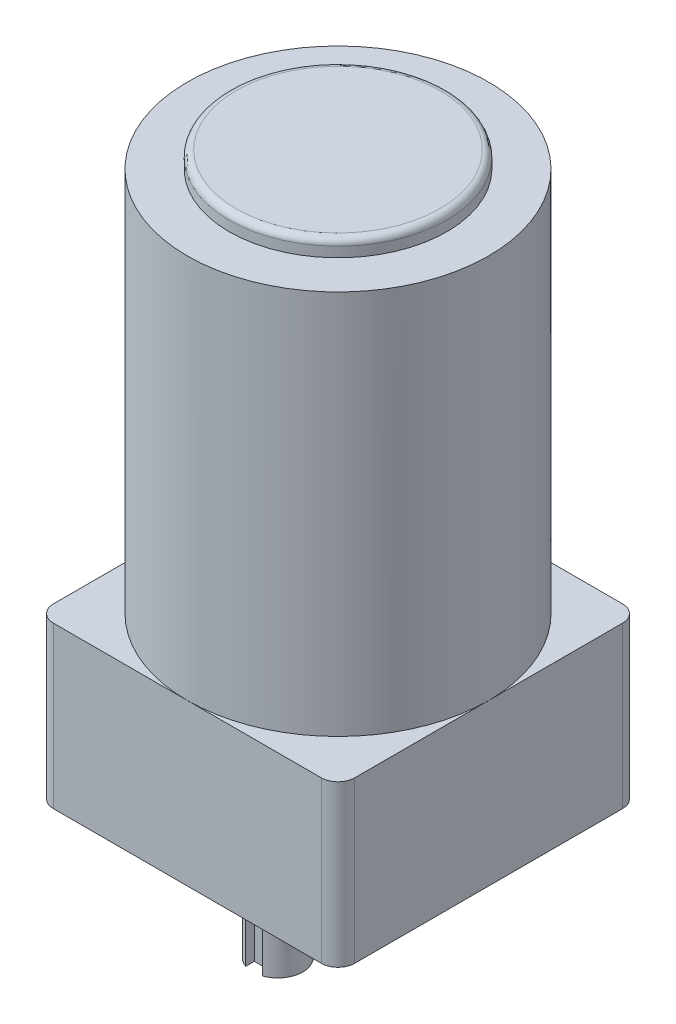
from build123d import *

# Parameters (mm, degrees)
SKETCH_1_W               = 90
SKETCH_1_H               = 90
EXTRUDE_1_DEPTH          = 43
SKETCH_2_R               = 18
EXTRUDE_2_DEPTH          = 3
SKETCH_3_R               = 7.5
EXTRUDE_3_DEPTH          = 29
CUT_EXTRUDE_1_DEPTH      = 3
PATTERN_CIRCULAR_1_COUNT = 4
SKETCH_8_R               = 45
EXTRUDE_4_DEPTH          = 120
SKETCH_9_R               = 32.5
EXTRUDE_5_DEPTH          = 5
SKETCH_10_W              = 90
SKETCH_10_H              = 90
EXTRUDE_6_DEPTH          = 5
FILLET_1_R               = 5
FILLET_2_R               = 2


with BuildPart() as part:
    # 草图1 → 凸台-拉伸1 (new body)
    with BuildSketch(Plane(origin=(0, 0, 0), x_dir=(1, 0, 0), z_dir=(0, 1, 0))):
        Rectangle(SKETCH_1_W, SKETCH_1_H)
    extrude(amount=EXTRUDE_1_DEPTH)

    # 草图2 → 凸台-拉伸2 (add)
    with BuildSketch(Plane.XZ):
        with Locations(Location((0, 18, 0), (0, 0, 90))):
            Circle(SKETCH_2_R)
    extrude(amount=EXTRUDE_2_DEPTH)

    # 草图3 → 凸台-拉伸3 (add)
    with BuildSketch(Plane.XZ.offset(3)):
        with Locations(Location((0, 18, 0), (0, 0, 90))):
            Circle(SKETCH_3_R)
    extrude(amount=EXTRUDE_3_DEPTH)

    # 草图4 → 切除-拉伸1 (cut)
    with BuildSketch(Plane.XY.offset(25.5)):
        with BuildLine():
            Line((-2.5, -7), (-2.5, -32))
            Line((-2.5, -32), (2.5, -32))
            Line((2.5, -32), (2.5, -7))
            ThreePointArc((2.5, -7), (0, -4.5), (-2.5, -7))
        make_face()
    extrude(amount=-CUT_EXTRUDE_1_DEPTH, mode=Mode.SUBTRACT)

    # 草图6 → M6x1.0 螺纹孔1 (revolve, cut)
    with BuildSketch(Plane(origin=(36.769552622, 0, 36.769552622), x_dir=(0, 0, -1), z_dir=(1, 0, 0))):
        Polygon((0, 0), (0, 18.502151548), (2.5, 17), (2.5, 0), align=None)
    m6x1_0_1 = revolve(axis=Axis((36.769552622, -6.35, 36.769552622), (0, 1, 0)), mode=Mode.SUBTRACT)

    # 阵列(圆周)1: M6x1.0 螺纹孔1 ×4 about axis
    pattern_circular_1_axis = Axis((0, 0, 0), (0, 1, 0))
    for i in range(1, PATTERN_CIRCULAR_1_COUNT):
        add(m6x1_0_1.rotate(pattern_circular_1_axis, i * 360 / PATTERN_CIRCULAR_1_COUNT), mode=Mode.SUBTRACT)

    # 草图8 → 凸台-拉伸4 (add)
    with BuildSketch(Plane(origin=(0, 43, 0), x_dir=(1, 0, 0), z_dir=(0, 1, 0))):
        with Locations(Location((0, 0, 0), (0, 0, 270))):
            Circle(SKETCH_8_R)
    extrude(amount=EXTRUDE_4_DEPTH)

    # 草图9 → 凸台-拉伸5 (add)
    with BuildSketch(Plane(origin=(0, 163, 0), x_dir=(1, 0, 0), z_dir=(0, 1, 0))):
        with Locations(Location((0, 0, 0), (0, 0, 270))):
            Circle(SKETCH_9_R)
    extrude(amount=EXTRUDE_5_DEPTH)

    # 草图10 → 凸台-拉伸6 (add)
    with BuildSketch(Plane(origin=(0, 43, 0), x_dir=(1, 0, 0), z_dir=(0, 1, 0))):
        Rectangle(SKETCH_10_W, SKETCH_10_H)
    extrude(amount=EXTRUDE_6_DEPTH)

    # 圆角1
    fillet_1_edges = [part.edges().sort_by_distance(p)[0] for p in [
        (-45, 24, -45),
        (45, 24, -45),
        (45, 24, 45),
        (-45, 24, 45),
    ]]
    fillet(fillet_1_edges, radius=FILLET_1_R)

    # 圆角2
    fillet_2_edges = [part.edges().sort_by_distance(p)[0] for p in [
        (0, 168, -32.5),
    ]]
    fillet(fillet_2_edges, radius=FILLET_2_R)


solid = part.part
